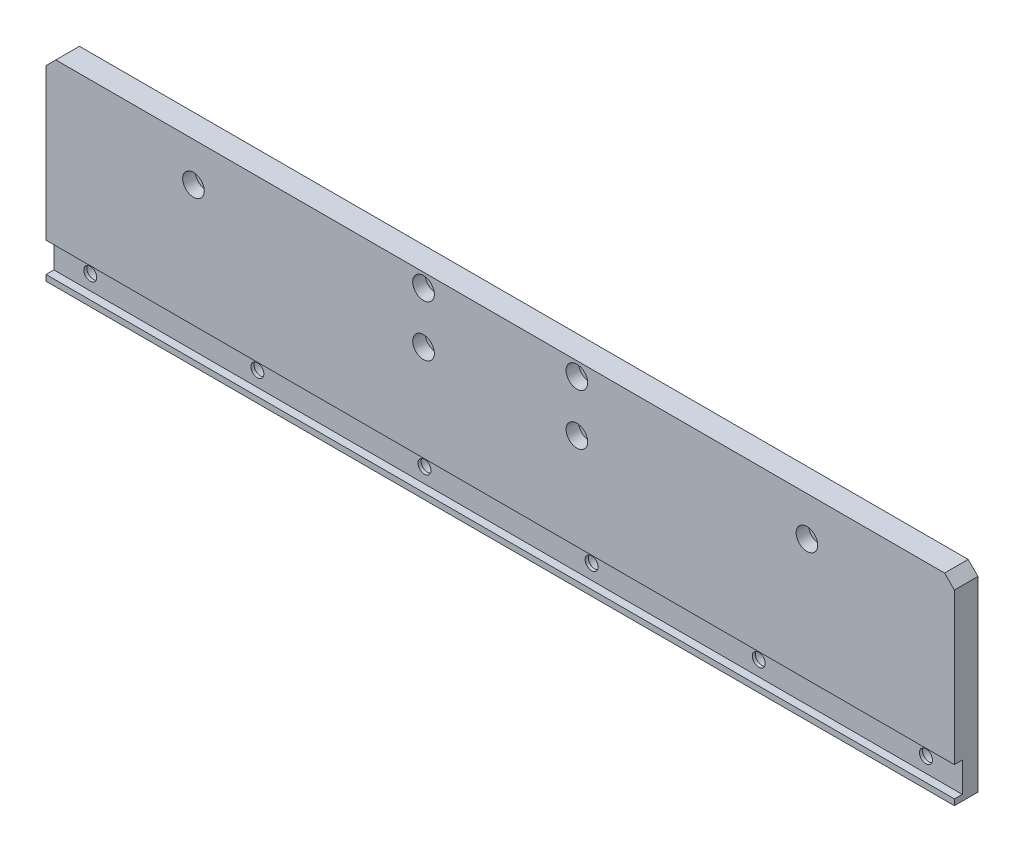
SolidWorks part; units mm, degrees
material "6061-T6"
ref_plane "前视基准面" through (0, 0, 0) normal (0, 0, 1) x (1, 0, 0)
ref_plane "上视基准面" through (0, 0, 0) normal (0, 1, 0) x (1, 0, 0)
ref_plane "右视基准面" through (0, 0, 0) normal (1, 0, 0) x (0, 0, -1)
sketch "草图1" plane through (0, 0, 0) normal (0, 0, 1) x (1, 0, 0)
  line L1 (0, 100) -> (462, 100)
  line L2 (0, 100) -> (0, 0)
  line L3 (0, 0) -> (462, 0)
  line L4 (462, 100) -> (462, 0)
  dimension "D1" = 462
  dimension "D2" = 100
extrude "凸台-拉伸1" add sketch "草图1" along normal blind 12
sketch "草图2" plane through (0, 0, 12) normal (0, 0, 1) x (1, 0, 0)
  line L0 (0, 100) -> (0, 0) construction
  line L1 (0, 18.1) -> (462, 18.1)
  line L2 (0, 18.1) -> (0, 3)
  line L3 (0, 3) -> (462, 3)
  line L4 (462, 18.1) -> (462, 3)
  line L5 (462, 0) -> (462, 100) construction
  line L6 (0, 0) -> (462, 0) construction
  dimension "D1" = 15.1
  dimension "D2" = 3
extrude "切除-拉伸1" cut sketch "草图2" against normal blind 4
hole_wizard "M6 六角凹头螺钉的柱形沉头孔1" positions "草图3" profile "草图4" counterbore size "M6" standard "ISO" end condition through all
sketch "草图3" plane through (0, 0, 12) normal (0, 0, 1) x (1, 0, 0)
  line L0 (192, 93) -> (270, 93) construction
  line L1 (270, 93) -> (270, 67) construction
  line L2 (270, 67) -> (192, 67) construction
  line L3 (192, 67) -> (192, 93) construction
  line L5 (462, 100) -> (0, 100) construction
  line L6 (231, 93) -> (231, 100) construction
  point P0 (192, 93)
  point P2 (270, 93)
  point P4 (192, 67)
  point P6 (270, 67)
  dimension "D1" = 78
  dimension "D2" = 26
  dimension "D3" = 7
sketch "草图4" plane through (192, 93, 12) normal (1, 0, 0) x (0, -1, 0)
  line L0 (0, 0) -> (0, 12)
  line L1 (0, 12) -> (3.3, 12)
  line L3 (3.3, 12) -> (3.3, 6.4)
  line L4 (3.3, 6.4) -> (5.5, 6.4)
  line L5 (5.5, 6.4) -> (5.5, 0)
  line L7 (5.5, 0) -> (0, 0)
  line L11 (0, -6.35) -> (0, 107.95) construction
  dimension "通孔孔直径" = 6.6
  dimension "通孔孔深度" = 12
  dimension "柱形沉头孔直径" = 11
  dimension "柱形沉头孔深度" = 6.4
sketch "草图5" plane through (0, 0, 0) normal (0, 0, -1) x (-1, 0, 0)
  line L0 (-75, 80) -> (-387, 80) construction
  line L1 (-231, 80) -> (-231, 100) construction
  line L2 (-462, 100) -> (0, 100) construction
  circle A0 centre (-387, 80) radius 10
  circle A1 centre (-75, 80) radius 10
  dimension "D2" = 20
  dimension "D1" = 312
  dimension "D3" = 20
extrude "切除-拉伸2" cut sketch "草图5" against normal blind 2
hole_wizard "M6 六角凹头螺钉的柱形沉头孔2" positions "草图6" profile "草图7" counterbore size "M6" standard "ISO" end condition through all
sketch "草图6" plane through (0, 0, 12) normal (0, 0, 1) x (1, 0, 0)
  line L0 (75, 80) -> (387, 80) construction
  line L2 (462, 100) -> (0, 100) construction
  line L3 (231, 80) -> (231, 100) construction
  point P0 (75, 80)
  point P2 (387, 80)
  dimension "D1" = 312
  dimension "D2" = 20
sketch "草图7" plane through (75, 80, 12) normal (1, 0, 0) x (0, -1, 0)
  line L0 (0, 0) -> (0, 12)
  line L1 (0, 12) -> (3.3, 12)
  line L3 (3.3, 12) -> (3.3, 6.4)
  line L4 (3.3, 6.4) -> (5.5, 6.4)
  line L5 (5.5, 6.4) -> (5.5, 0)
  line L7 (5.5, 0) -> (0, 0)
  line L11 (0, -6.35) -> (0, 107.95) construction
  dimension "通孔孔直径" = 6.6
  dimension "通孔孔深度" = 12
  dimension "柱形沉头孔直径" = 11
  dimension "柱形沉头孔深度" = 6.4
hole_wizard "M6 六角凹头螺钉的柱形沉头孔3" positions "草图10" profile "草图11" counterbore size "M6" standard "ISO" end condition through all
sketch "草图10" plane through (0, 0, 0) normal (0, 0, -1) x (-1, 0, 0)
  line L0 (-462, 18.1) -> (-462, 3) construction
  line L1 (-462, 18.1) -> (0, 18.1) construction
  line L2 (0, 3) -> (-462, 3) construction
  line L4 (-443.5, 10.55) -> (-462, 10.55) construction
  line L6 (-443.5, 10.55) -> (-18.5, 10.55) construction
  line L8 (-231, 10.55) -> (-231, 100) construction
  line L9 (-462, 100) -> (0, 100) construction
  line L10 (-462, 0) -> (-462, 100) construction
  point P0 (-443.5, 10.55)
  point P22 (-358.5, 10.55)
  point P23 (-273.5, 10.55)
  point P24 (-188.5, 10.55)
  point P25 (-103.5, 10.55)
  point P26 (-18.5, 10.55)
  dimension "D2" = 85
  dimension "D1" = 6
sketch "草图11" plane through (443.5, 10.55, 0) normal (1, 0, 0) x (0, 1, 0)
  line L0 (0, 0) -> (0, 12)
  line L1 (0, 12) -> (3.3, 12)
  line L3 (3.3, 12) -> (3.3, 6.4)
  line L4 (3.3, 6.4) -> (5.5, 6.4)
  line L5 (5.5, 6.4) -> (5.5, 0)
  line L7 (5.5, 0) -> (0, 0)
  line L11 (0, -6.35) -> (0, 107.95) construction
  dimension "通孔孔直径" = 6.6
  dimension "通孔孔深度" = 12
  dimension "柱形沉头孔直径" = 11
  dimension "柱形沉头孔深度" = 6.4
chamfer "倒角1" distance 5 angle 45 2 edges at (462, 100, 6) (0, 100, 6)
